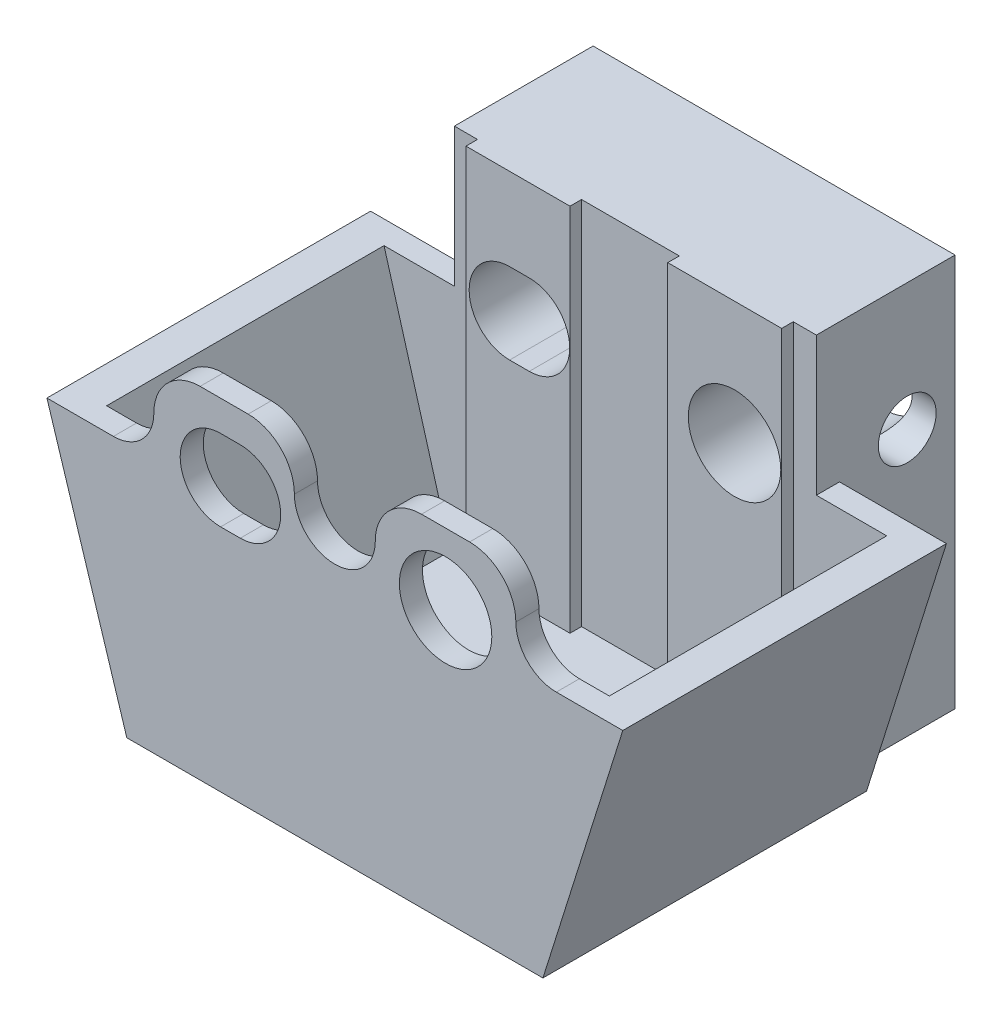
SolidWorks part; units mm, degrees
ref_plane "前视基准面" through (0, 0, 0) normal (0, 0, 1) x (1, 0, 0)
ref_plane "上视基准面" through (0, 0, 0) normal (0, 1, 0) x (1, 0, 0)
ref_plane "右视基准面" through (0, 0, 0) normal (1, 0, 0) x (0, 0, -1)
sketch "草图1" plane through (0, 0, 0) normal (0, 0, 1) x (1, 0, 0)
  line L0 (0, 0) -> (180, 0)
  line L1 (180, 0) -> (180, 220)
  line L2 (0, 0) -> (-69.0989, 220)
  line L3 (-69.0989, 220) -> (-11.5827, 220)
  line L4 (63.4173, 295) -> (105, 295)
  arc A0 (180, 220) -> (145, 255) centre (180, 255) cw
  arc A1 (-11.5827, 220) -> (23.4173, 255) centre (-11.5827, 255) ccw
  arc A2 (23.4173, 255) -> (63.4173, 295) centre (63.4173, 255) cw
  arc A3 (145, 255) -> (105, 295) centre (105, 255) ccw
extrude "凸台-拉伸2" add sketch "草图1" along normal blind 140
sketch3d "3D草图2"
  point P0 (98.2763, 115.3215, 0)
ref_plane "基准面2" through (0, 0, 0) normal (0, 0, -1) x (-1, 0, 0)
sketch "草图5" plane through (0, 0, 0) normal (0, 0, -1) x (-1, 0, 0)
  line L0 (-180, 220) -> (69.0989, 220)
  line L1 (69.0989, 220) -> (0, 0)
  line L2 (0, 0) -> (-180, 0)
  line L3 (-180, 0) -> (-180, 220)
extrude "凸台-拉伸3" add sketch "草图5" along normal blind 140
sketch3d "3D草图3"
  point P0 (84.2298, 295, 74.4461)
ref_plane "基准面3" through (0, 295, 0) normal (0, 1, 0) x (1, 0, 0)
sketch "草图8" plane through (0, 295, 0) normal (0, 1, 0) x (1, 0, 0)
  line L1 (180, -140) -> (180, 0) construction
  line L3 (180, 140) -> (180, 0) construction
  line L4 (180, 120) -> (80, 120)
  line L5 (80, 120) -> (80, -120)
  line L6 (80, -120) -> (180, -120)
  line L7 (180, 120) -> (180, -120)
extrude "切除-拉伸1" cut sketch "草图8" against normal blind 275
sketch3d "3D草图4"
  point P0 (116.3882, 20, -5.7324)
ref_plane "基准面4" through (0, 20, 0) normal (0, 1, 0) x (1, 0, 0)
sketch "草图10" plane through (0, 20, 0) normal (0, 1, 0) x (1, 0, 0)
  line L0 (80, 120) -> (20, 120)
  line L1 (20, 120) -> (20, -120)
  line L2 (20, -120) -> (80, -120)
  line L3 (80, -120) -> (80, 120)
sketch "草图11" plane through (0, 295, 0) normal (0, 1, 0) x (1, 0, 0)
  line L0 (80, 120) -> (80, -120)
  line L1 (80, -120) -> (-59, -120)
  line L2 (-59, -120) -> (-59, 120)
  line L3 (-59, 120) -> (80, 120)
loft "切除-放样4" cut profiles "草图10", "草图11"
mirror "镜向1" about plane through (180, 0, 140) normal (-1, 0, 0) of "切除-放样4", "切除-拉伸1", "凸台-拉伸3", "凸台-拉伸2"
sketch3d "3D草图5"
  point P0 (226.624, 136.3844, -140)
ref_plane "基准面5" through (0, 0, -140) normal (0, 0, -1) x (-1, 0, 0)
sketch "草图12" plane through (0, 0, -140) normal (0, 0, -1) x (-1, 0, 0)
  line L0 (-336.5827, 220) -> (-336.5827, 340)
  line L1 (69.0989, 220) -> (-429.0989, 220) construction
  line L2 (-336.5827, 220) -> (-23.4173, 220)
  line L3 (-336.5827, 340) -> (-23.4173, 340)
  line L4 (-23.4173, 340) -> (-23.4173, 220)
extrude "凸台-拉伸4" add sketch "草图12" along normal blind 100 and the other way blind 20
sketch "草图13" plane through (0, 0, -140) normal (0, 0, -1) x (-1, 0, 0)
  line L0 (-336.5827, 220) -> (-336.5827, 0)
  line L1 (-360, 0) -> (0, 0) construction
  line L2 (-336.5827, 0) -> (-23.4173, 0)
  line L3 (-23.4173, 0) -> (-23.4173, 220)
  line L4 (-23.4173, 220) -> (-336.5827, 220)
extrude "凸台-拉伸5" add sketch "草图13" along normal blind 100
sketch3d "3D草图6"
  point P0 (336.5827, 174.9086, -185.5314)
ref_plane "基准面6" through (336.5827, 0, 0) normal (1, 0, 0) x (0, 0, -1)
sketch "草图14" plane through (336.5827, 0, 0) normal (1, 0, 0) x (0, 0, -1)
  circle A0 centre (198.6209, 230) radius 25
  point P2 (0, 0)
extrude "切除-拉伸2" cut sketch "草图14" against normal through all
sketch3d "3D草图7"
  point P0 (201.9225, 340, -191.4158)
ref_plane "基准面7" through (0, 340, 0) normal (0, 1, 0) x (1, 0, 0)
sketch "草图15" plane through (0, 340, 0) normal (0, 1, 0) x (1, 0, 0)
  line L1 (23.4173, 120) -> (336.5827, 120) construction
  line L2 (43.4173, 120) -> (43.4173, 110)
  line L3 (43.4173, 110) -> (133.4173, 110)
  line L4 (133.4173, 110) -> (133.4173, 120)
  line L5 (280, 120) -> (80, 120) construction
  line L6 (133.4173, 120) -> (43.4173, 120)
  line L7 (316.5827, 120) -> (218, 120)
  line L8 (218, 120) -> (218, 110)
  line L9 (218, 110) -> (316.5827, 110)
  line L10 (316.5827, 110) -> (316.5827, 120)
extrude "凸台-拉伸6" add sketch "草图15" against normal up to surface (320 mm away) contours L2 L3 L4 L6 | L7 L8 L9 L10 up to face at (180, 20, -30)
sketch "草图16" plane through (0, 0, -140) normal (0, 0, -1) x (-1, 0, 0)
  line L2 (-98.1764, 268.6063) -> (-81.1764, 268.6063)
  line L3 (-81.1764, 198.6063) -> (-98.1764, 198.6063)
  circle A0 centre (-275.7914, 233.6063) radius 40
  arc A1 (-81.1764, 268.6063) -> (-81.1764, 198.6063) centre (-81.1764, 233.6063) cw
  arc A2 (-98.1764, 268.6063) -> (-98.1764, 198.6063) centre (-98.1764, 233.6063) ccw
extrude "切除-拉伸3" cut sketch "草图16" against normal through all both and the other way through all
